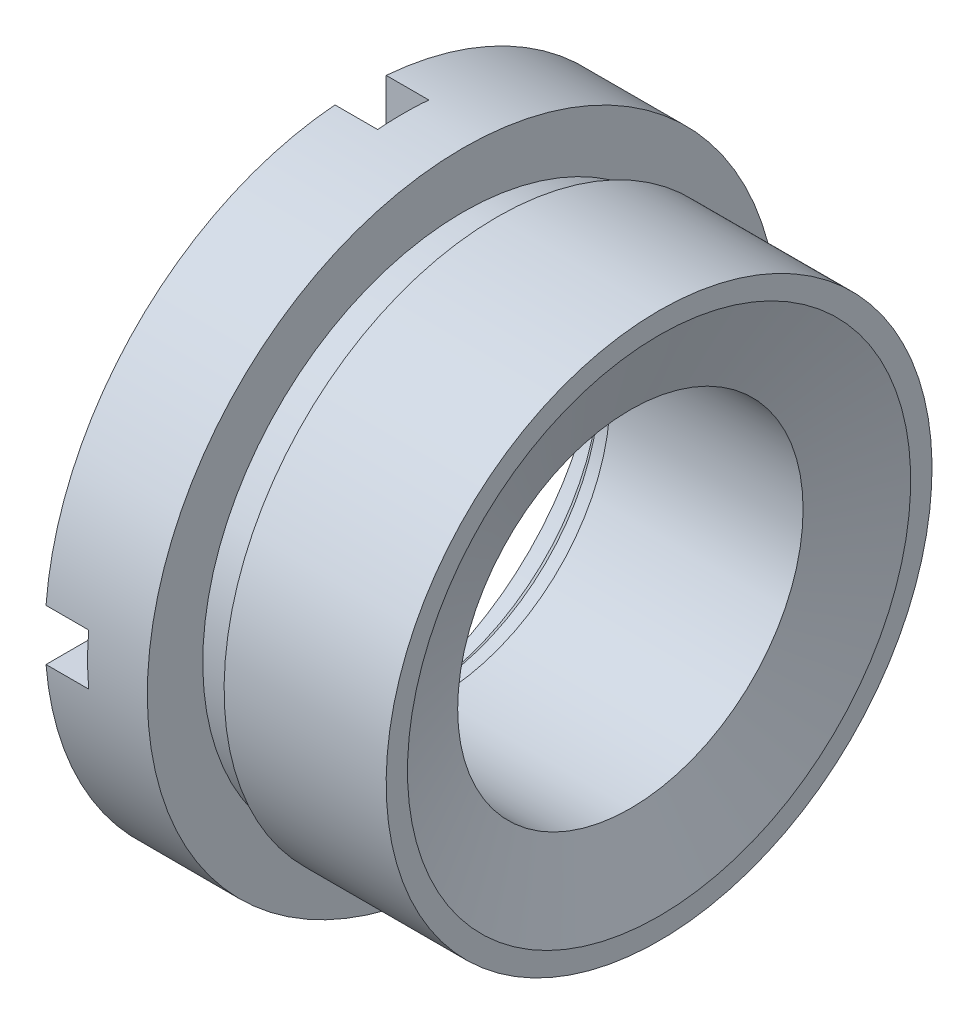
SolidWorks part; units mm, degrees
ref_plane "Front Plane" through (0, 0, 0) normal (0, 0, 1) x (1, 0, 0)
ref_plane "Top Plane" through (0, 0, 0) normal (0, 1, 0) x (1, 0, 0)
ref_plane "Right Plane" through (0, 0, 0) normal (1, 0, 0) x (0, 0, -1)
sketch "Sketch1" plane through (0, 0, 0) normal (0, 0, 1) x (1, 0, 0)
  line L0 (-23, 20.25) -> (-23, 32) construction
  line L5 (0, 0) -> (-23, 0)
  line L6 (0, 0) -> (0, 32)
  line L7 (0, 32) -> (-23, 32)
  line L8 (-23, 20.25) -> (-23, 32) construction
  line L9 (-23, 0) -> (-35, 0)
  line L10 (-23, 32) -> (-23, 37)
  line L11 (-23, 37) -> (-35, 37)
  line L12 (-35, 0) -> (-35, 37)
  line L13 (-23, 0) -> (-23, 20.25) construction
  line L14 (0, 0) -> (-3.3667, 0)
  line L15 (0, 0) -> (0, 29.5)
  line L16 (0, 29.5) -> (-3.3667, 20.25)
  line L17 (-3.3667, 0) -> (-3.3667, 20.25) construction
  line L18 (-3.3667, 0) -> (-26, 0)
  line L19 (-3.3667, 0) -> (-3.3667, 20.25) construction
  line L20 (-3.3667, 20.25) -> (-26, 20.25)
  line L21 (-26, 0) -> (-26, 20.25) construction
  line L30 (-26, 0) -> (-28, 0)
  line L31 (-26, 20.25) -> (-26, 21)
  line L32 (-26, 21) -> (-28, 21)
  line L33 (-28, 0) -> (-28, 21) construction
  line L34 (-28, 0) -> (-29, 0)
  line L35 (-28, 0) -> (-28, 21) construction
  line L36 (-28, 21) -> (-29, 22)
  line L37 (-29, 0) -> (-29, 22)
  line L38 (-29, 0) -> (-35, 0)
  line L39 (-29, 0) -> (-29, 28)
  line L40 (-29, 28) -> (-35, 28)
  line L41 (-35, 0) -> (-35, 28)
  line L42 (-23, 32) -> (-19, 32)
  line L43 (-23, 32) -> (-23, 30.5)
  line L44 (-23, 30.5) -> (-19, 30.5)
  line L45 (-19, 32) -> (-19, 30.5)
  line L46 (-23, 0) -> (-23, 20.25) construction
  line L47 (-26, 0) -> (-26, 20.25) construction
  dimension "D1" = 32
  dimension "D2" = 37
  dimension "D3" = 12
  dimension "D4" = 29.5
  dimension "D5" = 35
  dimension "D6" = 20.25
  dimension "D7" = 21
  dimension "D8" = 1
  dimension "D9" = 45
  dimension "D10" = 9
  dimension "D11" = 28
  dimension "D12" = 4
  dimension "D13" = 30.5
  dimension "D14" = 6
  dimension "D15" = 70
revolve "Revolve1" add sketch "Sketch1" angle 360 about L5
cosmetic thread "Cosmetic Thread1" parameters "D2"=57.505
sketch "Sketch2" plane through (-35, 0, 0) normal (-1, 0, 0) x (0, 0, 1)
  line L1 (-3, -53.3722) -> (3, -53.3722)
  line L2 (-3, -53.3722) -> (-3, 53.3722)
  line L3 (-3, 53.3722) -> (3, 53.3722)
  line L4 (3, -53.3722) -> (3, 53.3722)
  line L5 (-3, -53.3722) -> (3, 53.3722) construction
  line L6 (-3, 53.3722) -> (3, -53.3722) construction
  circle A1 centre (0, 0) radius 37
  circle A2 centre (0, 0) radius 37
  circle M1 centre (0, 0) radius 37
  circle M2 centre (0, 0) radius 28
  dimension "D2" = 6
  dimension "D1" = 0
extrude "Cut-Extrude1" cut sketch "Sketch2" against normal blind 5 contours L4 L2 M2 M1
pattern_circular "CirPattern1" count 4 over 360 about axis through (0, 0, 0) along (1, 0, 0) of "Cut-Extrude1"
